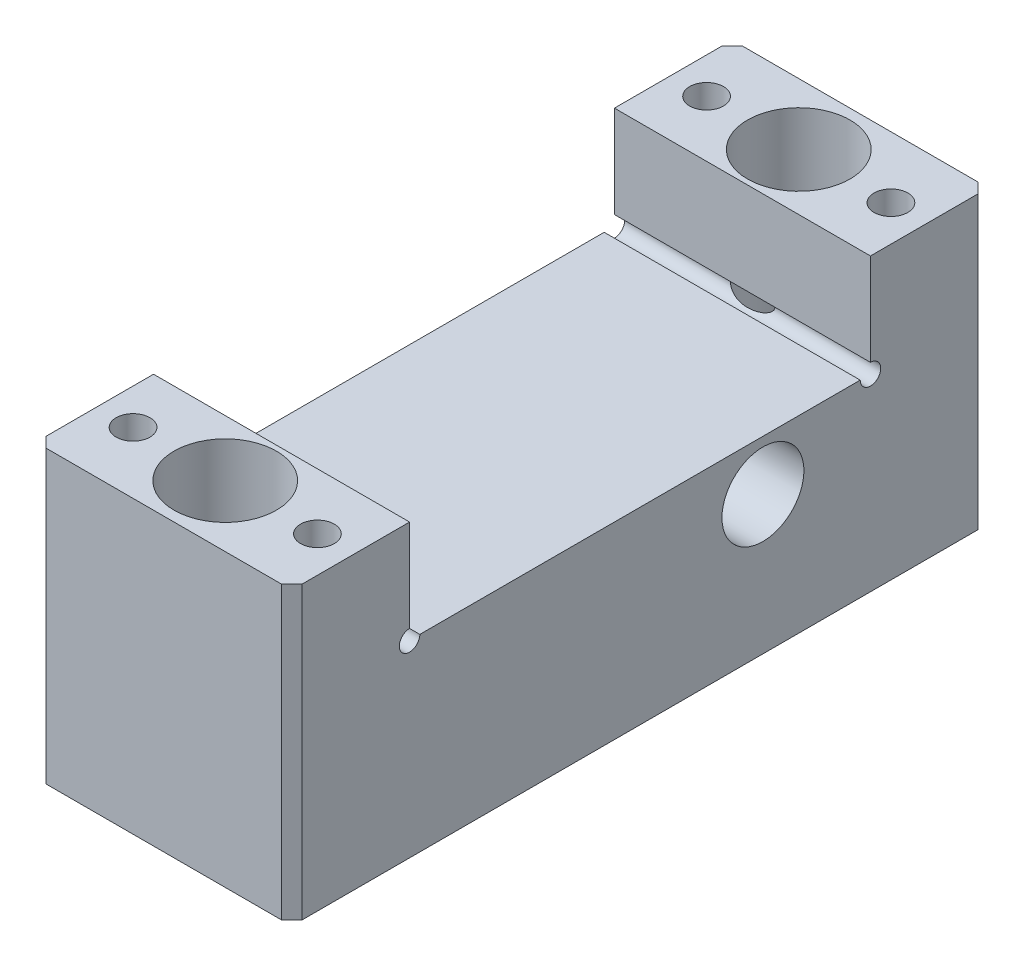
from build123d import *

# Parameters (mm, degrees)
SKETCH_1_W                   = 25
SKETCH_1_H                   = 68
EXTRUDE_1_DEPTH              = 14.2
CUT_EXTRUDE_1_DEPTH          = 47.030533345
CUT_EXTRUDE_1_DEPTH_BACK     = 10
SKETCH_2_W                   = 25
SKETCH_2_H                   = 45
F_6_0MM_1_D                  = 6
F_6_0MM_1_DEPTH              = 7
HOLE_WIZARD_M5_1_D           = 5.5
HOLE_WIZARD_M5_1_CBORE_D     = 10
HOLE_WIZARD_M5_1_CBORE_DEPTH = 20
HOLE_WIZARD_M4_1_D           = 3.3
HOLE_WIZARD_M4_1_DEPTH       = 10.1
HOLE_WIZARD_M4_1_TIP         = 0.991420021
CHAMFER_1_SIZE               = 1
SKETCH_9_R                   = 4
CUT_EXTRUDE_2_DEPTH          = 45.526845835
SKETCH_10_R                  = 1
CUT_EXTRUDE_3_DEPTH          = 45.526845835


with BuildPart() as part:
    # 草图1 → 凸台-拉伸1 (new, symmetric)
    with BuildSketch(Plane(origin=(0, 0, 0), x_dir=(1, 0, 0), z_dir=(0, 1, 0))):
        Rectangle(SKETCH_1_W, SKETCH_1_H)
    extrude(amount=EXTRUDE_1_DEPTH, both=True)

    # 草图2 → 切除-拉伸1 (cut, two sides: drawn at the far end of the back side and taken through both)
    with BuildSketch(Plane(origin=(0, 14.2, 0), x_dir=(1, 0, 0), z_dir=(0, 1, 0)).offset(-CUT_EXTRUDE_1_DEPTH_BACK)):
        Rectangle(SKETCH_2_W, SKETCH_2_H)
    extrude(amount=CUT_EXTRUDE_1_DEPTH + CUT_EXTRUDE_1_DEPTH_BACK, mode=Mode.SUBTRACT)

    # Ø6.0mm 暗销孔1
    with Locations(Plane(origin=(0, -14.2, 0), x_dir=(-1, 0, 0), z_dir=(0, -1, 0))):
        with Locations((0, 15), (0, -15)):
            Hole(F_6_0MM_1_D / 2, depth=F_6_0MM_1_DEPTH)

    # M5 六角凹头螺钉的柱形沉头孔1 (through all)
    with Locations(Plane(origin=(0, 14.2, 0), x_dir=(1, 0, 0), z_dir=(0, 1, 0))):
        with Locations((0, 28), (0, -28)):
            CounterBoreHole(HOLE_WIZARD_M5_1_D / 2, HOLE_WIZARD_M5_1_CBORE_D / 2, HOLE_WIZARD_M5_1_CBORE_DEPTH)

    # M4 螺纹孔1
    with Locations(Plane(origin=(0, 14.2, 0), x_dir=(1, 0, 0), z_dir=(0, 1, 0))):
        with Locations((-9, -28), (9, -28), (9, 28), (-9, 28)):
            Hole(HOLE_WIZARD_M4_1_D / 2, depth=HOLE_WIZARD_M4_1_DEPTH)
            with Locations((0, 0, -(HOLE_WIZARD_M4_1_DEPTH + HOLE_WIZARD_M4_1_TIP / 2))):  # 118° drill point
                Cone(0, HOLE_WIZARD_M4_1_D / 2, HOLE_WIZARD_M4_1_TIP, mode=Mode.SUBTRACT)

    # 倒角1
    chamfer_1_edges = [part.edges().sort_by_distance(p)[0] for p in [
        (12.5, 0, 34),
        (-12.5, 0, 34),
        (-12.5, 0, -34),
        (12.5, 0, -34),
    ]]
    chamfer(chamfer_1_edges, length=CHAMFER_1_SIZE)

    # 草图9 → 切除-拉伸2 (cut, through all)
    with BuildSketch(Plane.ZY.offset(12.5)):
        with Locations((-12, -0.7)):
            Circle(SKETCH_9_R)
    extrude(amount=-CUT_EXTRUDE_2_DEPTH, mode=Mode.SUBTRACT)

    # 草图10 → 切除-拉伸3 (cut, through all)
    with BuildSketch(Plane(origin=(12.5, 0, 0), x_dir=(0, 0, -1), z_dir=(1, 0, 0))):
        with Locations((-22.5, 4.2)):
            Circle(SKETCH_10_R)
        with Locations((22.5, 4.2)):
            Circle(SKETCH_10_R)
    extrude(amount=-CUT_EXTRUDE_3_DEPTH, mode=Mode.SUBTRACT)


solid = part.part
